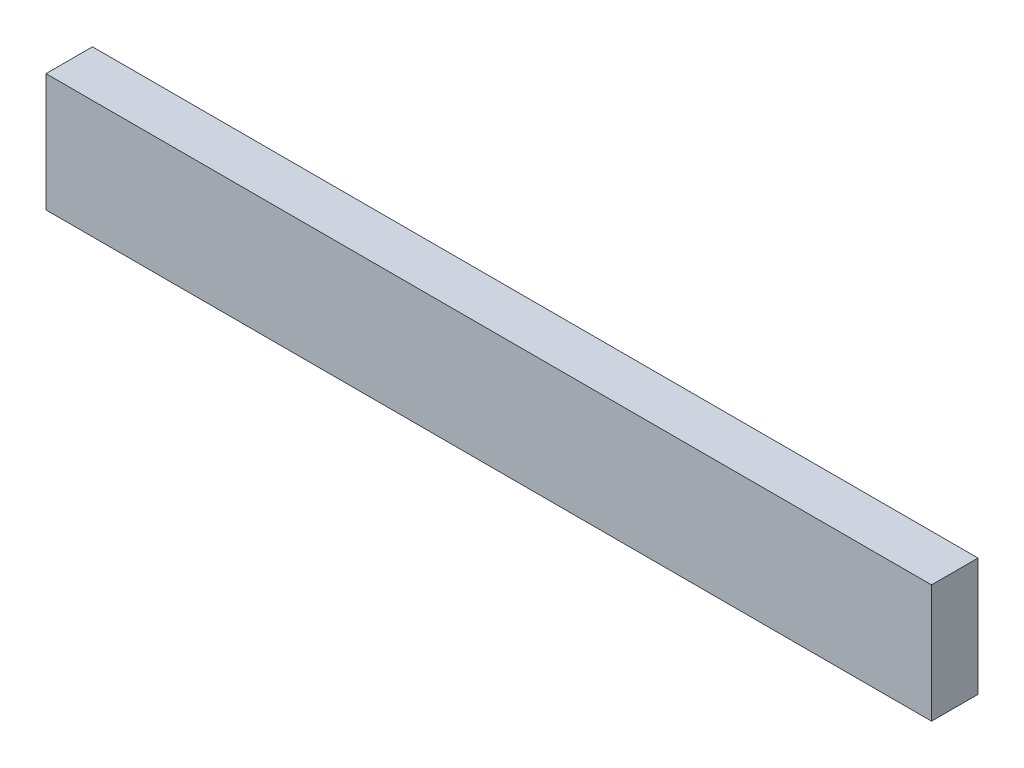
SolidWorks part; units mm, degrees
material "普通碳钢"
ref_plane "Front Plane" through (0, 0, 0) normal (0, 0, 1) x (1, 0, 0)
ref_plane "Top Plane" through (0, 0, 0) normal (0, 1, 0) x (1, 0, 0)
ref_plane "Right Plane" through (0, 0, 0) normal (1, 0, 0) x (0, 0, -1)
sketch "Sketch1" plane through (0, 0, 0) normal (0, 0, 1) x (1, 0, 0)
  line L1 (-95.25, 12.7) -> (95.25, 12.7)
  line L2 (-95.25, 12.7) -> (-95.25, -12.7)
  line L3 (-95.25, -12.7) -> (95.25, -12.7)
  line L4 (95.25, 12.7) -> (95.25, -12.7)
  dimension "D1" = 190.5
  dimension "D2" = 95.25
  dimension "D3" = 25.4
  dimension "D4" = 12.7
extrude "Boss-Extrude1" add sketch "Sketch1" along normal mid plane 10
